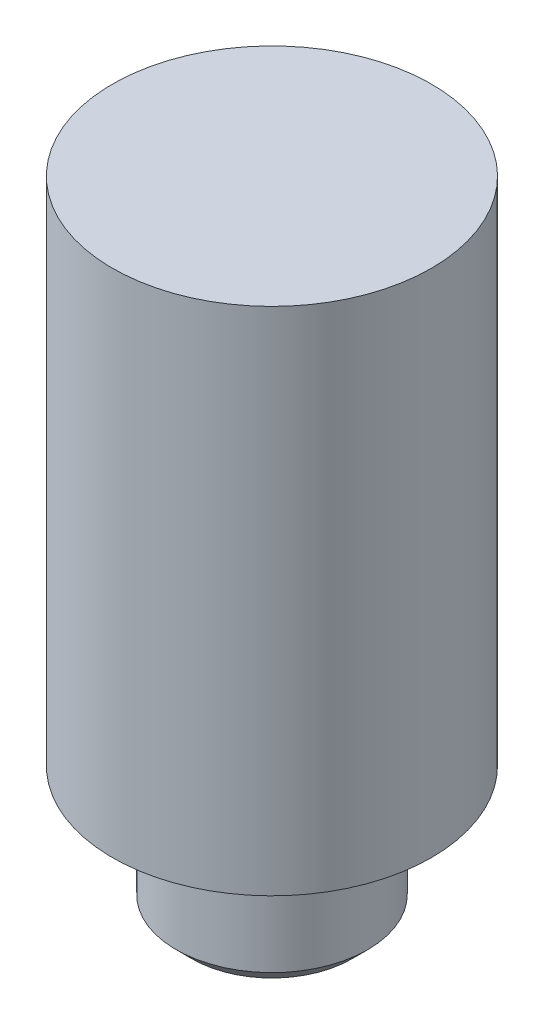
from build123d import *

# Parameters (mm, degrees)
CHAMFER2_SIZE = 0.5


with BuildPart() as part:
    # Sketch1 → Revolve1 (revolve)
    with BuildSketch(Plane.XY):
        Polygon((0, 0), (5, 0), (5, -16), (3, -16), (3, -20), (0, -20), align=None)
    revolve(axis=Axis((0, -324.964502388, 0), (0, 1, 0)))

    # Chamfer2
    chamfer2_edges = [part.edges().sort_by_distance(p)[0] for p in [
        (-3, -20, 0),
    ]]
    chamfer(chamfer2_edges, length=CHAMFER2_SIZE)


solid = part.part
